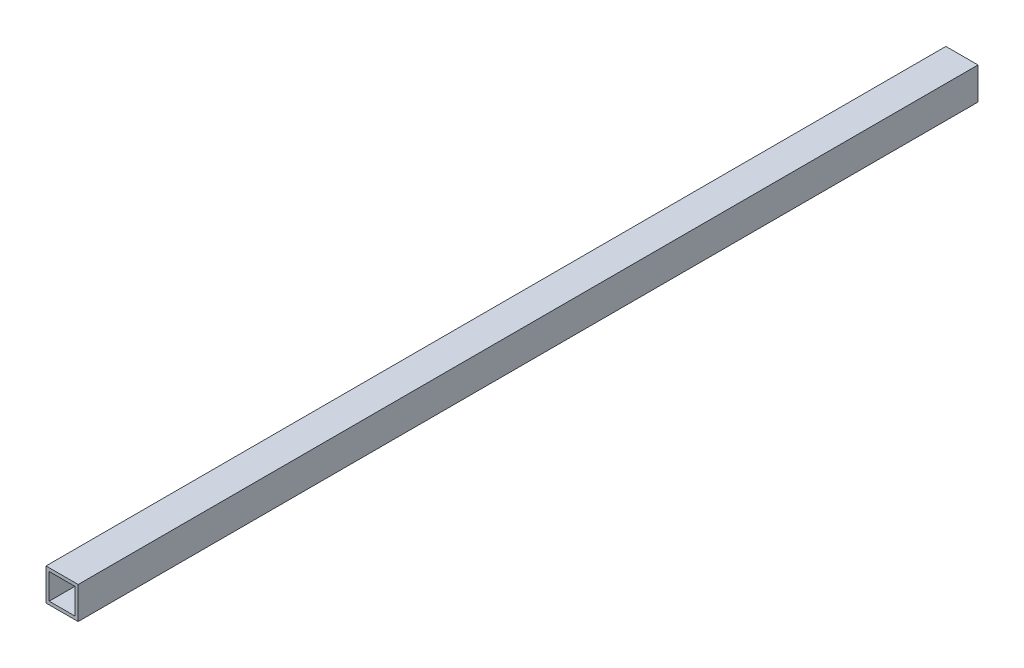
SolidWorks part; units mm, degrees
ref_plane "Front Plane" through (0, 0, 0) normal (0, 0, 1) x (1, 0, 0)
ref_plane "Top Plane" through (0, 0, 0) normal (0, 1, 0) x (1, 0, 0)
ref_plane "Right Plane" through (0, 0, 0) normal (1, 0, 0) x (0, 0, -1)
other "Configuration Table"
sketch "Sketch1" plane through (0, 0, 0) normal (0, 0, 1) x (1, 0, 0)
  line L0 (-11.1328, 32.3444) -> (18.8672, 32.3444)
  line L1 (18.8672, 32.3444) -> (18.8672, 2.3444)
  line L2 (18.8672, 2.3444) -> (-11.1328, 2.3444)
  line L3 (-11.1328, 2.3444) -> (-11.1328, 32.3444)
  dimension "D1" = 30
  dimension "D2" = 30
extrude "Boss-Extrude1" add sketch "Sketch1" along normal blind 840
sketch "Sketch2" plane through (0, 0, 840) normal (0, 0, 1) x (1, 0, 0)
  line L0 (-8.1328, 29.3444) -> (15.8672, 29.3444)
  line L1 (15.8672, 29.3444) -> (15.8672, 5.3444)
  line L2 (15.8672, 5.3444) -> (-8.1328, 5.3444)
  line L3 (-8.1328, 5.3444) -> (-8.1328, 29.3444)
  line L4 (18.8672, 2.3444) -> (18.8672, 32.3444) construction
  line L5 (18.8672, 32.3444) -> (-11.1328, 32.3444) construction
  line L6 (-11.1328, 2.3444) -> (18.8672, 2.3444) construction
  line L7 (-11.1328, 32.3444) -> (-11.1328, 2.3444) construction
  dimension "D1" = 3
  dimension "D2" = 3
  dimension "D3" = 3
  dimension "D4" = 3
extrude "Cut-Extrude1" cut sketch "Sketch2" against normal blind 840
